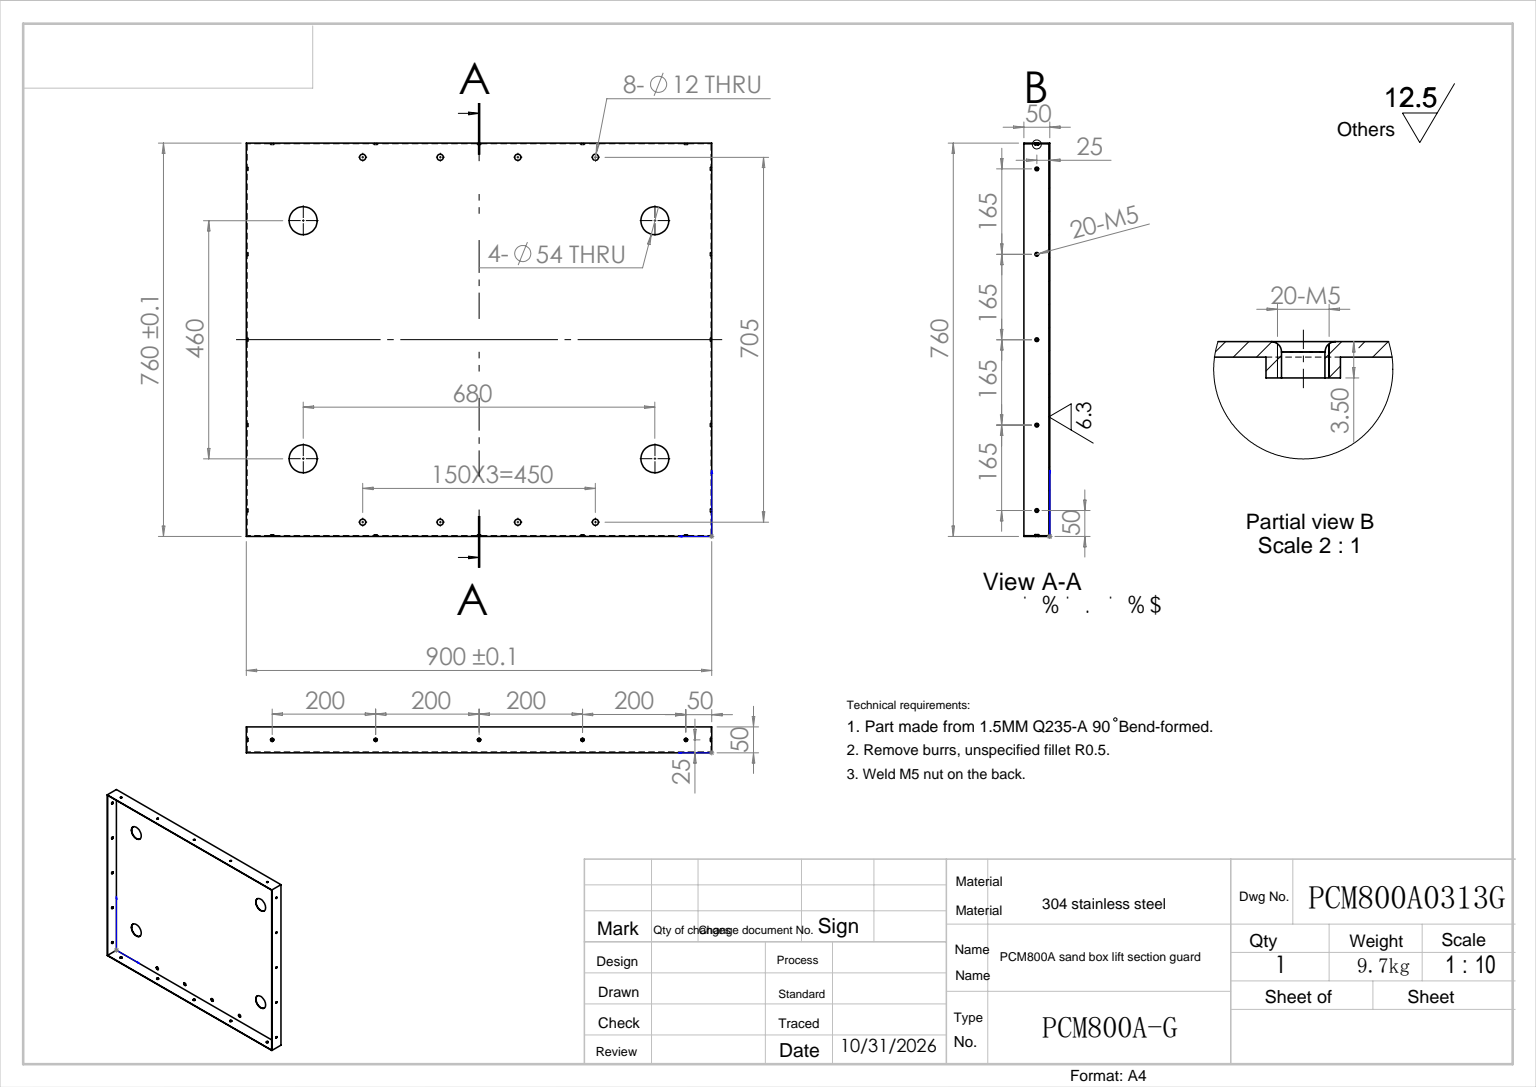
from build123d import *

# Parameters (mm, degrees)
SKETCH_1_W          = 900
SKETCH_1_H          = 760
EXTRUDE_1_DEPTH     = 50
SHELL_1_T           = -1.5
SKETCH_2_R          = 27
CUT_EXTRUDE_1_DEPTH = 1180.025020939
SKETCH_3_R          = 6
CUT_EXTRUDE_3_DEPTH = 1180.025020939
SKETCH_6_R          = 3.6
EXTRUDE_1_2_DEPTH   = 2
EXTRUDE_START       = 2
SKETCH_7_R          = 3.6
EXTRUDE_2_DEPTH     = 2
HOLE_WIZARD_M5_1_D  = 4.2
SKETCH_10_R         = 3.6
EXTRUDE_3_DEPTH     = 2
SKETCH_11_R         = 3.6
EXTRUDE_4_DEPTH     = 2
HOLE_WIZARD_M5_2_D  = 4.2
FILLET_1_R          = 1


with BuildPart() as part:
    # 草图1 → Extrude 1 (new body)
    with BuildSketch(Plane.XY):
        with Locations((450, 380)):
            Rectangle(SKETCH_1_W, SKETCH_1_H)
    extrude(amount=EXTRUDE_1_DEPTH)

    # 抽壳1
    shell_1_openings = [part.faces().sort_by_distance(p)[0] for p in [
        (450, 380, 50),
    ]]
    offset(amount=SHELL_1_T, openings=shell_1_openings, kind=Kind.INTERSECTION)

    # 草图2 → 切除-拉伸1 (cut, through all)
    with BuildSketch(Plane(origin=(0, 0, 0), x_dir=(-1, 0, 0), z_dir=(0, 0, -1))):
        with Locations((-790, 610)):
            Circle(SKETCH_2_R)
        with Locations((-110, 610)):
            Circle(SKETCH_2_R)
        with Locations((-790, 150)):
            Circle(SKETCH_2_R)
        with Locations((-110, 150)):
            Circle(SKETCH_2_R)
    extrude(amount=-CUT_EXTRUDE_1_DEPTH, mode=Mode.SUBTRACT)

    # 草图3 → 切除-拉伸3 (cut, through all)
    with BuildSketch(Plane(origin=(0, 0, 0), x_dir=(-1, 0, 0), z_dir=(0, 0, -1))):
        with Locations((-675, 732.5)):
            Circle(SKETCH_3_R)
        with Locations((-525, 732.5)):
            Circle(SKETCH_3_R)
        with Locations((-375, 732.5)):
            Circle(SKETCH_3_R)
        with Locations((-225, 732.5)):
            Circle(SKETCH_3_R)
    cut_extrude_3 = extrude(amount=-CUT_EXTRUDE_3_DEPTH, mode=Mode.SUBTRACT)

    # 镜向1: 切除-拉伸3 across plane
    add(cut_extrude_3.mirror(Plane.ZX.offset(380)), mode=Mode.SUBTRACT)

    # 草图6 → Extrude 1 2 (add)
    with BuildSketch(Plane(origin=(0, 1.5, 0), x_dir=(1, 0, 0), z_dir=(0, 1, 0))):
        with Locations(Location((50, -25, 0), (0, 0, 270))):
            Circle(SKETCH_6_R)
        with Locations(Location((250, -25, 0), (0, 0, 270))):
            Circle(SKETCH_6_R)
        with Locations(Location((450, -25, 0), (0, 0, 270))):
            Circle(SKETCH_6_R)
        with Locations(Location((650, -25, 0), (0, 0, 270))):
            Circle(SKETCH_6_R)
        with Locations(Location((850, -25, 0), (0, 0, 270))):
            Circle(SKETCH_6_R)
    extrude(amount=EXTRUDE_1_2_DEPTH)

    # 草图7 → 凸台-拉伸2 (add)
    with BuildSketch(Plane.XZ.offset(-758.5).offset(EXTRUDE_START)):
        with Locations(Location((50, 25, 0), (0, 0, 90))):
            Circle(SKETCH_7_R)
        with Locations(Location((250, 25, 0), (0, 0, 90))):
            Circle(SKETCH_7_R)
        with Locations(Location((450, 25, 0), (0, 0, 90))):
            Circle(SKETCH_7_R)
        with Locations(Location((650, 25, 0), (0, 0, 90))):
            Circle(SKETCH_7_R)
        with Locations(Location((850, 25, 0), (0, 0, 90))):
            Circle(SKETCH_7_R)
    extrude(amount=-EXTRUDE_2_DEPTH)

    # M5 螺纹孔1 (through all)
    with Locations(Plane.XZ):
        with Locations((50, 25), (250, 25), (450, 25), (650, 25), (850, 25)):
            Hole(HOLE_WIZARD_M5_1_D / 2)

    # 草图10 → 凸台-拉伸3 (add)
    with BuildSketch(Plane(origin=(1.5, 0, 0), x_dir=(0, 0, -1), z_dir=(1, 0, 0))):
        with Locations((-25, 710)):
            Circle(SKETCH_10_R)
        with Locations((-25, 545)):
            Circle(SKETCH_10_R)
        with Locations((-25, 380)):
            Circle(SKETCH_10_R)
        with Locations((-25, 215)):
            Circle(SKETCH_10_R)
        with Locations((-25, 50)):
            Circle(SKETCH_10_R)
    extrude(amount=EXTRUDE_3_DEPTH)

    # 草图11 → 凸台-拉伸4 (add)
    with BuildSketch(Plane.ZY.offset(-898.5).offset(EXTRUDE_START)):
        with Locations(Location((25, 710, 0), (0, 0, 180))):
            Circle(SKETCH_11_R)
        with Locations(Location((25, 545, 0), (0, 0, 180))):
            Circle(SKETCH_11_R)
        with Locations(Location((25, 380, 0), (0, 0, 180))):
            Circle(SKETCH_11_R)
        with Locations(Location((25, 215, 0), (0, 0, 180))):
            Circle(SKETCH_11_R)
        with Locations(Location((25, 50, 0), (0, 0, 180))):
            Circle(SKETCH_11_R)
    extrude(amount=-EXTRUDE_4_DEPTH)

    # M5 螺纹孔2 (through all)
    with Locations(Plane(origin=(900, 0, 0), x_dir=(0, 0, -1), z_dir=(1, 0, 0))):
        with Locations((-25, 710), (-25, 545), (-25, 380), (-25, 215), (-25, 50)):
            Hole(HOLE_WIZARD_M5_2_D / 2)

    # 圆角1
    fillet_1_edges = [part.edges().sort_by_distance(p)[0] for p in [
        (852.1, 760, 25),
        (852.1, 0, 25),
        (652.1, 0, 25),
        (652.1, 760, 25),
        (452.1, 0, 25),
        (452.1, 760, 25),
        (252.1, 0, 25),
        (252.1, 760, 25),
        (52.1, 0, 25),
        (52.1, 760, 25),
        (0, 50, 22.9),
        (900, 50, 22.9),
        (0, 215, 22.9),
        (900, 215, 22.9),
        (0, 380, 22.9),
        (900, 380, 22.9),
        (0, 545, 22.9),
        (900, 545, 22.9),
        (0, 710, 22.9),
        (900, 710, 22.9),
    ]]
    fillet(fillet_1_edges, radius=FILLET_1_R)


solid = part.part
